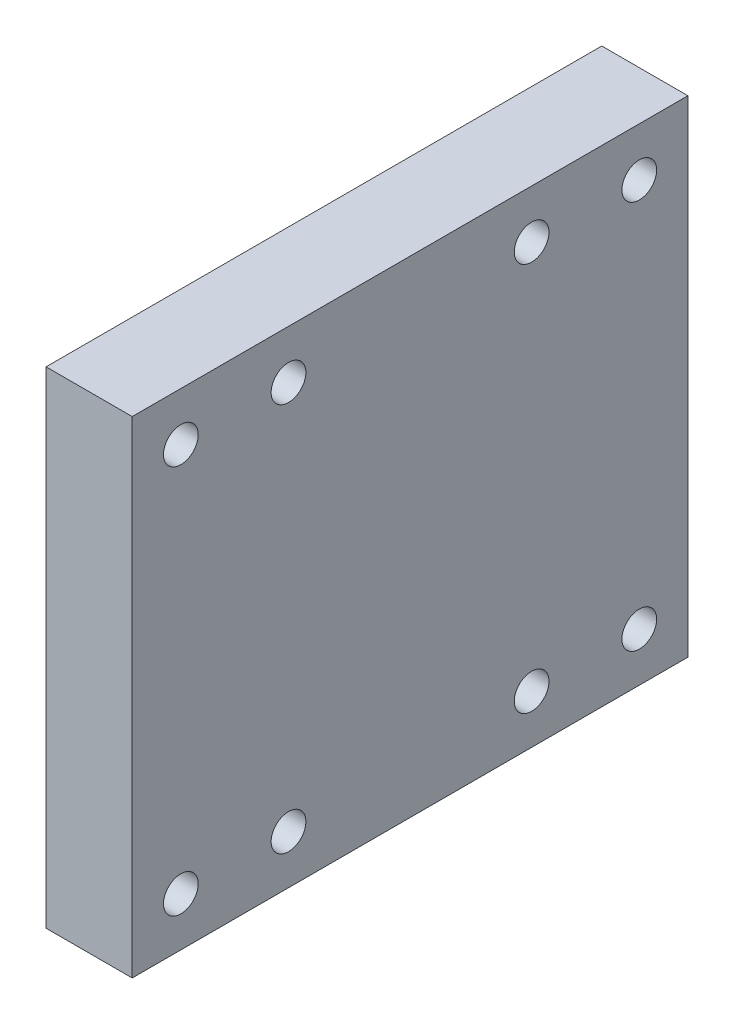
from build123d import *

# Parameters (mm, degrees)
SKETCH_1_W             = 80
SKETCH_1_H             = 70
EXTRUDE_1_DEPTH        = 12.4
HOLE_WIZARD_M6_1_D     = 5
HOLE_WIZARD_M6_1_DEPTH = 15
HOLE_WIZARD_M6_1_TIP   = 1.502151548
HOLE_WIZARD_M6_2_D     = 5


with BuildPart() as part:
    # 草图1 → 凸台-拉伸1 (new body)
    with BuildSketch(Plane(origin=(0, 0, 0), x_dir=(0, 0, -1), z_dir=(1, 0, 0))):
        Rectangle(SKETCH_1_W, SKETCH_1_H)
    extrude(amount=EXTRUDE_1_DEPTH)

    # M6 螺纹孔1
    with Locations(Plane(origin=(12.4, 0, 0), x_dir=(0, 0, -1), z_dir=(1, 0, 0))):
        with Locations((-17.5, 28), (17.5, 28), (-17.5, -28), (17.5, -28)):
            Hole(HOLE_WIZARD_M6_1_D / 2, depth=HOLE_WIZARD_M6_1_DEPTH)
            with Locations((0, 0, -(HOLE_WIZARD_M6_1_DEPTH + HOLE_WIZARD_M6_1_TIP / 2))):  # 118° drill point
                Cone(0, HOLE_WIZARD_M6_1_D / 2, HOLE_WIZARD_M6_1_TIP, mode=Mode.SUBTRACT)

    # M6 螺纹孔2 (through all)
    with Locations(Plane(origin=(12.4, 0, 0), x_dir=(0, 0, -1), z_dir=(1, 0, 0))):
        with Locations((-33, 28), (-33, -28), (33, -28), (33, 28)):
            Hole(HOLE_WIZARD_M6_2_D / 2)


solid = part.part
